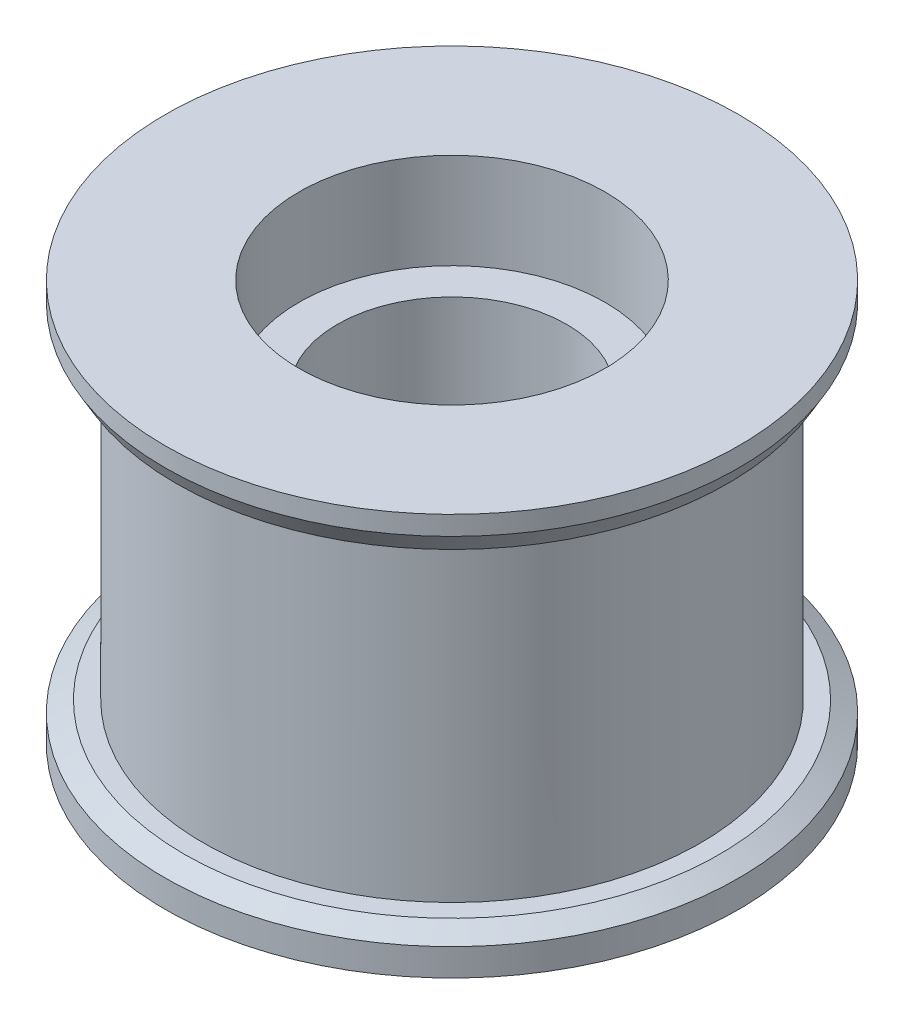
SolidWorks part; units mm, degrees
material "6061 合金"
ref_plane "前视基准面" through (0, 0, 0) normal (0, 0, 1) x (1, 0, 0)
ref_plane "上视基准面" through (0, 0, 0) normal (0, 1, 0) x (1, 0, 0)
ref_plane "右视基准面" through (0, 0, 0) normal (1, 0, 0) x (0, 0, -1)
sketch "草图1" plane through (0, 0, 0) normal (0, 0, 1) x (1, 0, 0)
  line L0 (0, 0) -> (0, 32.2299) construction
  line L1 (6, -10.5) -> (6, 10.5)
  line L2 (0, 0) -> (6, 0) construction
  line L4 (6, 10.5) -> (12.99, 10.5)
  line L5 (12.99, 10.5) -> (12.99, -10.5)
  line L6 (12.99, -10.5) -> (6, -10.5)
  dimension "D1" = 21
  dimension "D3" = 12
  dimension "D4" = 25.98
revolve "旋转1" add sketch "草图1" angle 360 about L0
sketch "草图4" plane through (0, -10.5, 0) normal (0, -1, 0) x (1, 0, 0)
  circle A0 centre (0, 0) radius 8
  dimension "D1" = 16
extrude "切除-拉伸3" cut sketch "草图4" against normal blind 5
sketch "草图5" plane through (0, -10.5, 0) normal (0, -1, 0) x (1, 0, 0)
  circle A0 centre (0, 0) radius 8 construction
  circle A1 centre (0, 0) radius 15
  circle A3 centre (0, 0) radius 8
  dimension "D1" = 30
extrude "凸台-拉伸1" add sketch "草图5" against normal blind 2
mirror "镜向1" about plane through (0, 0, 0) normal (0, 1, 0) of "凸台-拉伸1", "切除-拉伸3"
chamfer "倒角1" distance 1 angle 30 1 edges at (0, 8.5, -15)
chamfer "倒角2" distance 1 angle 30 1 edges at (0, -8.5, -15)
